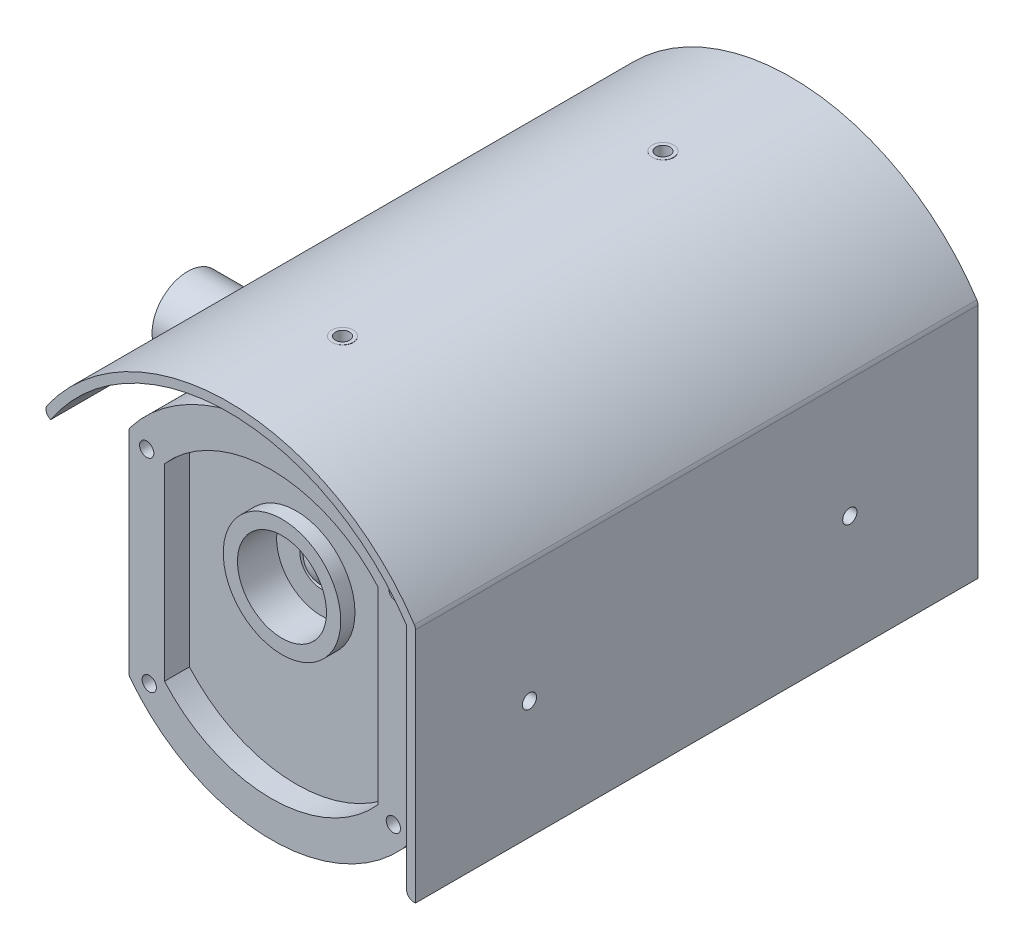
from build123d import *

# Parameters (mm, degrees)
BOSS_EXTRUDE1_DEPTH      = 140
CUT_EXTRUDE1_DEPTH       = 7
BOSS_EXTRUDE2_DEPTH      = 12
BOSS_EXTRUDE2_DEPTH_BACK = 146
SKETCH4_R                = 16.5
SKETCH4_R_2              = 12.5
BOSS_EXTRUDE3_DEPTH      = 4
CUT_EXTRUDE2_START       = -7
SKETCH5_R                = 12.5
CUT_EXTRUDE2_DEPTH       = 7
SKETCH6_R                = 6
CUT_EXTRUDE3_DEPTH       = 1
DOME1_FACE_RADIUS        = 6
DOME1_HEIGHT             = 3
SKETCH7_R                = 3
BOSS_EXTRUDE4_DEPTH      = 12.5
SKETCH8_R                = 2
CUT_EXTRUDE4_DEPTH       = 17
BOSS_EXTRUDE5_REACH      = 198.256
BOSS_EXTRUDE5_END_RADIUS = 50
SKETCH9_R                = 3
SKETCH10_R               = 2
CUT_EXTRUDE5_DEPTH       = 17
BOSS_EXTRUDE6_DEPTH      = 7
SKETCH12_W               = 70
SKETCH12_H               = 3.5
CUT_EXTRUDE6_DEPTH       = 5
SKETCH13_R               = 10
BOSS_EXTRUDE7_DEPTH      = 50
SKETCH14_R               = 15
SKETCH14_R_2             = 10
BOSS_EXTRUDE8_DEPTH      = 20
FILLET1_R                = 2
SKETCH15_R               = 2
CUT_EXTRUDE7_DEPTH       = 5
SCALE1_SCALE             = 0.5


with BuildPart() as part:
    # Sketch1 → Boss-Extrude1 (new body)
    with BuildSketch(Plane.XY):
        with BuildLine():
            Line((-40, -30), (-40, 30))
            ThreePointArc((-40, 30), (0, 50), (40, 30))
            Line((40, 30), (40, -30))
            ThreePointArc((40, -30), (0, -50), (-40, -30))
        make_face()
    extrude(amount=BOSS_EXTRUDE1_DEPTH)

    # Sketch2 → Cut-Extrude1 (cut)
    with BuildSketch(Plane.XY.offset(140)):
        with BuildLine():
            Line((-30, 26.457513111), (-30, -26.457513111))
            ThreePointArc((-30, -26.457513111), (0, -40), (30, -26.457513111))
            Line((30, -26.457513111), (30, 26.457513111))
            ThreePointArc((30, 26.457513111), (0, 40), (-30, 26.457513111))
        make_face()
    extrude(amount=-CUT_EXTRUDE1_DEPTH, mode=Mode.SUBTRACT)

    # Sketch4 → Boss-Extrude3 (add)
    with BuildSketch(Plane.XY.offset(133)):
        with Locations((0, 10)):
            Circle(SKETCH4_R)
        with Locations((0, 10)):
            Circle(SKETCH4_R_2, mode=Mode.SUBTRACT)
    extrude(amount=BOSS_EXTRUDE3_DEPTH)

    # Sketch5 → Cut-Extrude2 (cut)
    with BuildSketch(Plane.XY.offset(133).offset(CUT_EXTRUDE2_START)):
        with Locations((0, 10)):
            Circle(SKETCH5_R)
    extrude(amount=CUT_EXTRUDE2_DEPTH, mode=Mode.SUBTRACT)

    # Sketch6 → Cut-Extrude3 (cut)
    with BuildSketch(Plane.XY.offset(126)):
        with Locations((0, 10)):
            Circle(SKETCH6_R)
    extrude(amount=-CUT_EXTRUDE3_DEPTH, mode=Mode.SUBTRACT)

    # Dome1: a dome of height H over a round flat face of radius A is a cap of a sphere of radius (A * A + H * H) / (2 * H)
    dome1_r = (DOME1_FACE_RADIUS * DOME1_FACE_RADIUS + DOME1_HEIGHT * DOME1_HEIGHT) / (2 * DOME1_HEIGHT)
    dome1_base = Plane((0, 10, 125), z_dir=(0, 0, 1))
    with Locations(dome1_base.offset(DOME1_HEIGHT - dome1_r)):
        dome1_ball = Sphere(dome1_r, mode=Mode.PRIVATE)
    add(split(dome1_ball, bisect_by=dome1_base, keep=Keep.TOP, mode=Mode.PRIVATE))



with BuildPart() as body_2:
    # Sketch3 → Boss-Extrude2 (new, two sides: drawn at the far end of the back side and taken through both)
    with BuildSketch(Plane.XY.offset(140).offset(-BOSS_EXTRUDE2_DEPTH_BACK)):
        with BuildLine():
            Line((52.5, -33.166247904), (52.5, 33.911649916))
            ThreePointArc((52.5, 33.911649916), (0.380386371, 62.498842439), (-52.083333333, 34.5481749))
            Line((-52.083333333, 34.5481749), (-50, 33.166247904))
            ThreePointArc((-50, 33.166247904), (0, 60), (50, 33.166247904))
            Line((50, 33.166247904), (50, -33.166247904))
            Line((50, -33.166247904), (52.5, -33.166247904))
        make_face()
    extrude(amount=BOSS_EXTRUDE2_DEPTH + BOSS_EXTRUDE2_DEPTH_BACK)


with BuildPart() as part_1:
    add(part.part)

    add(body_2.part)  # Boss-Extrude4 merges body 2
    # Sketch7 → Boss-Extrude4 (add)
    with BuildSketch(Plane(origin=(52.5, 0, 0), x_dir=(0, 0, -1), z_dir=(1, 0, 0))):
        with Locations(Location((-120, 0, 0), (0, 0, 270))):
            Circle(SKETCH7_R)
        with Locations(Location((-30, 0, 0), (0, 0, 270))):
            Circle(SKETCH7_R)
    extrude(amount=-BOSS_EXTRUDE4_DEPTH)

    # Sketch8 → Cut-Extrude4 (cut)
    with BuildSketch(Plane(origin=(52.5, 0, 0), x_dir=(0, 0, -1), z_dir=(1, 0, 0))):
        with Locations((-120, 0)):
            Circle(SKETCH8_R)
        with Locations((-30, 0)):
            Circle(SKETCH8_R)
    extrude(amount=-CUT_EXTRUDE4_DEPTH, mode=Mode.SUBTRACT)

    # Boss-Extrude5: up to this cylinder (the profile starts outside it)
    boss_extrude5_end = Plane(origin=(0, 0, 75), z_dir=(0, 0, -1)) * Cylinder(BOSS_EXTRUDE5_END_RADIUS, 587.512, mode=Mode.PRIVATE)
    # Sketch9 → Boss-Extrude5 (add, up to the surface)
    with BuildSketch(Plane(origin=(0, 62.5, 0), x_dir=(-1, 0, 0), z_dir=(0, 1, 0)), mode=Mode.PRIVATE) as boss_extrude5_sk1:
        with Locations(Location((0, 120, 0), (0, 0, 90))):
            Circle(SKETCH9_R)
    boss_extrude5_tool1 = extrude(boss_extrude5_sk1.sketch, amount=-BOSS_EXTRUDE5_REACH, mode=Mode.PRIVATE) - boss_extrude5_end
    add(boss_extrude5_tool1.solids().sort_by_distance((0, 62.5, 120))[0])
    # Sketch9 → Boss-Extrude5 (add, up to the surface)
    with BuildSketch(Plane(origin=(0, 62.5, 0), x_dir=(-1, 0, 0), z_dir=(0, 1, 0)), mode=Mode.PRIVATE) as boss_extrude5_sk2:
        with Locations(Location((0, 30, 0), (0, 0, 90))):
            Circle(SKETCH9_R)
    boss_extrude5_tool2 = extrude(boss_extrude5_sk2.sketch, amount=-BOSS_EXTRUDE5_REACH, mode=Mode.PRIVATE) - boss_extrude5_end
    add(boss_extrude5_tool2.solids().sort_by_distance((0, 62.5, 30))[0])

    # Sketch10 → Cut-Extrude5 (cut)
    with BuildSketch(Plane(origin=(0, 62.5, 0), x_dir=(1, 0, 0), z_dir=(0, 1, 0))):
        with Locations(Location((0, -30, 0), (0, 0, 270))):
            Circle(SKETCH10_R)
        with Locations(Location((0, -120, 0), (0, 0, 270))):
            Circle(SKETCH10_R)
    extrude(amount=-CUT_EXTRUDE5_DEPTH, mode=Mode.SUBTRACT)

    # Sketch11 → Boss-Extrude6 (add)
    with BuildSketch(Plane(origin=(0, 0, 0), x_dir=(-1, 0, 0), z_dir=(0, 0, -1))):
        with BuildLine():
            Line((-42, 30.659419434), (-42, -30.659419434))
            ThreePointArc((-42, -30.659419434), (0, -52), (42, -30.659419434))
            Line((42, -30.659419434), (42, 30.659419434))
            ThreePointArc((42, 30.659419434), (0, 52), (-42, 30.659419434))
        make_face()
        with BuildLine():
            Line((-40, 30), (-40, -30))
            ThreePointArc((-40, -30), (0, -50), (40, -30))
            Line((40, -30), (40, 30))
            ThreePointArc((40, 30), (0, 50), (-40, 30))
        make_face(mode=Mode.SUBTRACT)
    extrude(amount=-BOSS_EXTRUDE6_DEPTH)

    # Sketch12 → Cut-Extrude6 (cut)
    with BuildSketch(Plane(origin=(0, 0, 0), x_dir=(-1, 0, 0), z_dir=(0, 0, -1))):
        with BuildLine():
            ThreePointArc((16.155494421, 42), (0, 45), (-16.155494421, 42))
            Line((-16.155494421, 42), (16.155494421, 42))
        make_face()
        with BuildLine():
            ThreePointArc((-21.558061137, 39.5), (-24.342017693, 37.84793488), (-27, 36))
            Line((-27, 36), (27, 36))
            ThreePointArc((27, 36), (24.342017693, 37.84793488), (21.558061137, 39.5))
            Line((21.558061137, 39.5), (-21.558061137, 39.5))
        make_face()
        with BuildLine():
            ThreePointArc((-30.045798375, 33.5), (-31.841535092, 31.798060365), (-33.541019662, 30))
            Line((-33.541019662, 30), (33.541019662, 30))
            ThreePointArc((33.541019662, 30), (31.841535092, 31.798060365), (30.045798375, 33.5))
            Line((30.045798375, 33.5), (-30.045798375, 33.5))
        make_face()
        with Locations((0, 25.75)):
            Rectangle(SKETCH12_W, SKETCH12_H)
        with Locations((0, 19.75)):
            Rectangle(SKETCH12_W, SKETCH12_H)
        with Locations((0, 13.75)):
            Rectangle(SKETCH12_W, SKETCH12_H)
        with Locations((0, 7.75)):
            Rectangle(SKETCH12_W, SKETCH12_H)
        with Locations((0, 1.75)):
            Rectangle(SKETCH12_W, SKETCH12_H)
        with Locations((0, -4.25)):
            Rectangle(SKETCH12_W, SKETCH12_H)
        with Locations((0, -10.25)):
            Rectangle(SKETCH12_W, SKETCH12_H)
        with Locations((0, -16.25)):
            Rectangle(SKETCH12_W, SKETCH12_H)
        with Locations((0, -22.25)):
            Rectangle(SKETCH12_W, SKETCH12_H)
        with BuildLine():
            Line((35, -26.5), (-35, -26.5))
            Line((-35, -26.5), (-35, -28.284271247))
            ThreePointArc((-35, -28.284271247), (-34.281245243, -29.151264546), (-33.541019662, -30))
            Line((-33.541019662, -30), (33.541019662, -30))
            ThreePointArc((33.541019662, -30), (34.281245243, -29.151264546), (35, -28.284271247))
            Line((35, -28.284271247), (35, -26.5))
        make_face()
        with BuildLine():
            Line((31.124748995, -32.5), (-31.124748995, -32.5))
            ThreePointArc((-31.124748995, -32.5), (-29.115015223, -34.31203708), (-27, -36))
            Line((-27, -36), (27, -36))
            ThreePointArc((27, -36), (29.115015223, -34.31203708), (31.124748995, -32.5))
        make_face()
        with BuildLine():
            Line((23.296995514, -38.5), (-23.296995514, -38.5))
            ThreePointArc((-23.296995514, -38.5), (-19.803717846, -40.408077899), (-16.155494421, -42))
            Line((-16.155494421, -42), (16.155494421, -42))
            ThreePointArc((16.155494421, -42), (19.803717846, -40.408077899), (23.296995514, -38.5))
        make_face()
    extrude(amount=-CUT_EXTRUDE6_DEPTH, mode=Mode.SUBTRACT)

    # Sketch13 → Boss-Extrude7 (add)
    with BuildSketch(Plane.ZY.offset(40)):
        with Locations(Location((73.5, 0, 0), (0, 0, 90))):
            Circle(SKETCH13_R)
    extrude(amount=BOSS_EXTRUDE7_DEPTH)

    # Sketch14 → Boss-Extrude8 (add)
    with BuildSketch(Plane.ZY.offset(40)):
        with Locations(Location((73.5, 0, 0), (0, 0, 90))):
            Circle(SKETCH14_R)
        with Locations(Location((73.5, 0, 0), (0, 0, 270))):
            Circle(SKETCH14_R_2, mode=Mode.SUBTRACT)
    extrude(amount=BOSS_EXTRUDE8_DEPTH)

    # Fillet1
    fillet1_edges = [part_1.edges().sort_by_distance(p)[0] for p in [
        (50, -33.166247904, 73),
        (-52.083333333, 34.5481749, 73),
        (52.5, 33.911649916, 73),
        (42, 30.659419434, 3.5),
        (-42, 30.659419434, 3.5),
        (-42, -30.659419434, 3.5),
        (42, -30.659419434, 3.5),
        (0, 52, 0),
        (42, 0, 0),
        (0, -52, 0),
        (-42, 0, 0),
        (-40, -15, 73.5),
        (50, 3, 120),
        (40, 3, 120),
        (40, 30, 73.5),
        (-40, 30, 73.5),
        (-40, -30, 73.5),
        (40, -30, 73.5),
        (50, 3, 30),
        (40, 3, 30),
        (-2e-09, 60.000000006, 117.000000018),
        (-2e-09, 50.000000007, 117.000000018),
        (0, 59.999999997, 26.999999988),
        (0, 49.999999997, 26.999999988),
    ]]
    fillet(fillet1_edges, radius=FILLET1_R)

    # Sketch15 → Cut-Extrude7 (cut)
    with BuildSketch(Plane.XY.offset(140)):
        with Locations((35, 27.5)):
            Circle(SKETCH15_R)
        with Locations((-35, 27.5)):
            Circle(SKETCH15_R)
        with Locations((34.281245243, -29.151264546)):
            Circle(SKETCH15_R)
        with Locations((-34.281245243, -29.151264546)):
            Circle(SKETCH15_R)
    extrude(amount=-CUT_EXTRUDE7_DEPTH, mode=Mode.SUBTRACT)


with BuildPart() as part_2:
    # Scale1: scaled about (0, 0, 0)
    add(part_1.part.scale(SCALE1_SCALE))


solid = part_2.part
